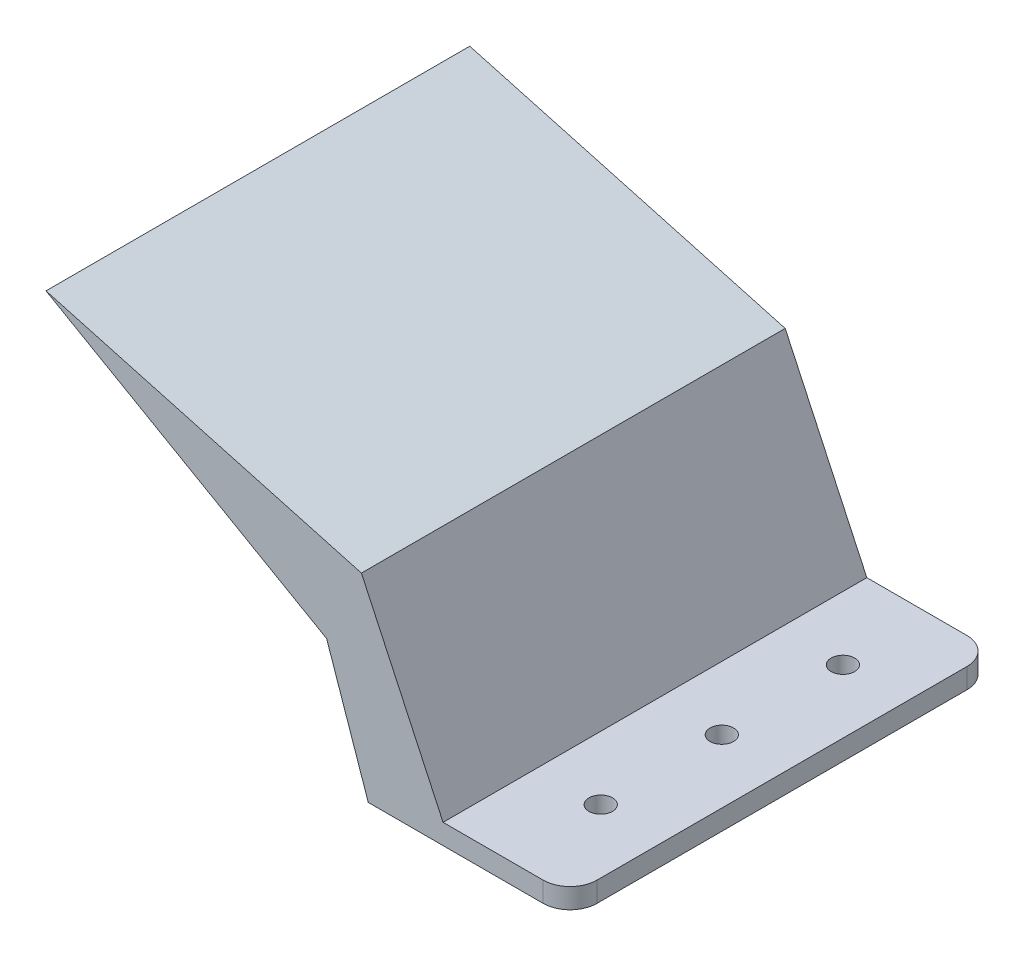
from build123d import *

# Parameters (mm, degrees)
BOSS_EXTRUDE1_DEPTH = 31.5
SKETCH2_W           = 30
SKETCH2_H           = 3
BOSS_EXTRUDE2_DEPTH = 63
SKETCH3_R           = 1.75
CUT_EXTRUDE1_DEPTH  = 50
FILLET1_R           = 4


with BuildPart() as part:
    # Sketch1 → Boss-Extrude1 (new, symmetric)
    with BuildSketch(Plane.XY):
        Polygon((0, 0), (-6.189633375, 18), (-47.911924672, 41.911648908), (-1.016937138, 29.024958443), (12.517623262, 0), align=None)
    extrude(amount=BOSS_EXTRUDE1_DEPTH, both=True)

    # Sketch2 → Boss-Extrude2 (add)
    with BuildSketch(Plane.XY.offset(31.5)):
        with Locations((15, 1.5)):
            Rectangle(SKETCH2_W, SKETCH2_H)
    extrude(amount=-BOSS_EXTRUDE2_DEPTH)

    # Sketch3 → Cut-Extrude1 (cut)
    with BuildSketch(Plane(origin=(0, 3, 0), x_dir=(1, 0, 0), z_dir=(0, 1, 0))):
        with Locations(Location((20.559350144, 18.5, 0), (0, 0, 270))):
            Circle(SKETCH3_R)
        with Locations(Location((20.559350144, 0.5, 0), (0, 0, 270))):
            Circle(SKETCH3_R)
        with Locations(Location((20.559350144, -17.5, 0), (0, 0, 270))):
            Circle(SKETCH3_R)
    extrude(amount=-CUT_EXTRUDE1_DEPTH, mode=Mode.SUBTRACT)

    # Fillet1
    fillet1_edges = [part.edges().sort_by_distance(p)[0] for p in [
        (30, 1.5, 31.5),
        (30, 1.5, -31.5),
    ]]
    fillet(fillet1_edges, radius=FILLET1_R)


solid = part.part
